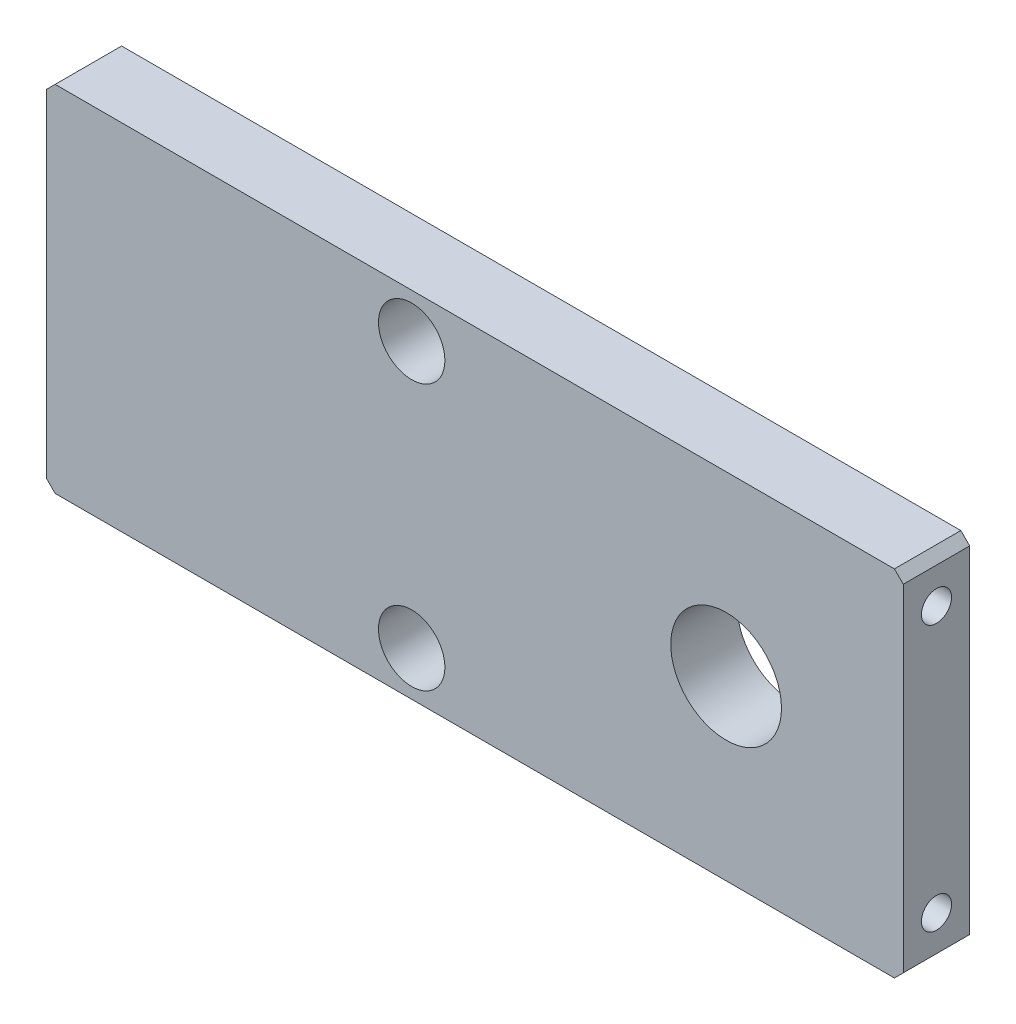
SolidWorks part; units mm, degrees
ref_plane "前视基准面" through (0, 0, 0) normal (0, 0, 1) x (1, 0, 0)
ref_plane "上视基准面" through (0, 0, 0) normal (0, 1, 0) x (1, 0, 0)
ref_plane "右视基准面" through (0, 0, 0) normal (1, 0, 0) x (0, 0, -1)
sketch "草图1" plane through (0, 0, 0) normal (0, 0, 1) x (1, 0, 0)
  line L1 (-96.75, 40) -> (96.75, 40)
  line L2 (-96.75, 40) -> (-96.75, -40)
  line L3 (-96.75, -40) -> (96.75, -40)
  line L4 (96.75, 40) -> (96.75, -40)
  line L5 (-96.75, 40) -> (96.75, -40) construction
  line L6 (-96.75, -40) -> (96.75, 40) construction
  point P0 (0, 0)
  dimension "D1" = 193.5
  dimension "D2" = 80
extrude "凸台-拉伸1" add sketch "草图1" along normal mid plane 15
hole_wizard "Ø25.0 (25) 直径孔1" positions "草图3" profile "草图2" hole size "Ø25.0" standard "ISO" end condition through all
sketch "草图3" plane through (0, 0, 7.5) normal (0, 0, 1) x (1, 0, 0)
  line L0 (96.75, -40) -> (96.75, 40) construction
  line L1 (-96.75, -40) -> (96.75, -40) construction
  point P0 (56.75, 0)
  dimension "D1" = 40
  dimension "D2" = 40
sketch "草图2" plane through (56.75, 0, 7.5) normal (1, 0, 0) x (0, -1, 0)
  line L0 (0, 0) -> (0, 15)
  line L1 (0, 15) -> (12.5, 15)
  line L2 (12.5, 15) -> (12.5, 0)
  line L5 (12.5, 0) -> (0, 0)
  line L11 (0, -6.35) -> (0, 107.95) construction
  dimension "通孔孔直径" = 25
  dimension "通孔孔深度" = 15
hole_wizard "Ø15.0 (15) 直径孔1" positions "草图5" profile "草图4" hole size "Ø15.0" standard "ISO" end condition through all
sketch "草图5" plane through (0, 0, 7.5) normal (0, 0, 1) x (1, 0, 0)
  line L0 (-96.75, 40) -> (-96.75, -40) construction
  point P0 (-14.25, 30)
  point P2 (-14.25, -30)
  dimension "D1" = 82.5
  dimension "D2" = 60
  dimension "D3" = 30
sketch "草图4" plane through (-14.25, 30, 7.5) normal (1, 0, 0) x (0, -1, 0)
  line L0 (0, 0) -> (0, 15)
  line L1 (0, 15) -> (7.5, 15)
  line L2 (7.5, 15) -> (7.5, 0)
  line L5 (7.5, 0) -> (0, 0)
  line L11 (0, -6.35) -> (0, 107.95) construction
  dimension "通孔孔直径" = 15
  dimension "通孔孔深度" = 15
hole_wizard "M8 螺纹孔1" positions "草图7" profile "草图6" tap size "M8" standard "ISO"
sketch "草图7" plane through (96.75, 0, 0) normal (1, 0, 0) x (0, 0, -1)
  line L0 (-7.5, -40) -> (7.5, -40) construction
  point P0 (0, 30)
  point P2 (0, -30)
  dimension "D1" = 60
  dimension "D2" = 10
sketch "草图6" plane through (96.75, 30, 0) normal (0, 1, 0) x (0, 0, -1)
  line L0 (0, 0) -> (0, 21.7929)
  line L1 (0, 21.7929) -> (3.4, 19.75)
  line L2 (3.4, 19.75) -> (3.4, 0)
  line L5 (3.4, 0) -> (0, 0)
  line L10 (0, 21.7929) -> (-3.4, 19.75) construction
  line L11 (0, -6.35) -> (0, 107.95) construction
  dimension "螺纹孔钻头直径" = 6.8
  dimension "螺纹孔钻头深度" = 19.75
  dimension "导头角度" = 118
cosmetic thread "孔螺蚊线1" parameters "D1"=16, "D2"=8
cosmetic thread "孔螺蚊线2" parameters "D1"=16, "D2"=8
hole_wizard "M8 螺纹孔2" positions "草图9" profile "草图8" tap size "M8" standard "ISO"
sketch "草图9" plane through (-96.75, 0, 0) normal (-1, 0, 0) x (0, 0, 1)
  line L0 (7.5, -40) -> (-7.5, -40) construction
  point P0 (0, 30)
  point P2 (0, -30)
  point P7 (0, -40)
  dimension "D1" = 60
  dimension "D2" = 10
sketch "草图8" plane through (-96.75, 30, 0) normal (0, 1, 0) x (0, 0, 1)
  line L0 (0, 0) -> (0, 21.7929)
  line L1 (0, 21.7929) -> (3.4, 19.75)
  line L2 (3.4, 19.75) -> (3.4, 0)
  line L5 (3.4, 0) -> (0, 0)
  line L10 (0, 21.7929) -> (-3.4, 19.75) construction
  line L11 (0, -6.35) -> (0, 107.95) construction
  dimension "螺纹孔钻头直径" = 6.8
  dimension "螺纹孔钻头深度" = 19.75
  dimension "导头角度" = 118
cosmetic thread "孔螺蚊线3" parameters "D1"=16, "D2"=8
cosmetic thread "孔螺蚊线4" parameters "D1"=16, "D2"=8
sketch "草图11" plane through (-96.75, 0, 0) normal (-1, 0, 0) x (0, 0, 1)
  line L0 (11.1757, 0) -> (-63.8976, 0) construction
  line L1 (-52.5, 18.9763) -> (-52.5, -18.6643) construction
  line L2 (-7.5, 40) -> (-7.5, -40) construction
  circle A0 centre (-52.5, 0) radius 56
  dimension "D2" = 112
  dimension "D1" = 45
extrude "切除-拉伸1" cut sketch "草图11" against normal blind 10
chamfer "倒角1" distance 2 angle 45 4 edges at (-96.75, 40, 0) (-96.75, -40, 0) (96.75, -40, 0) (96.75, 40, 0)
